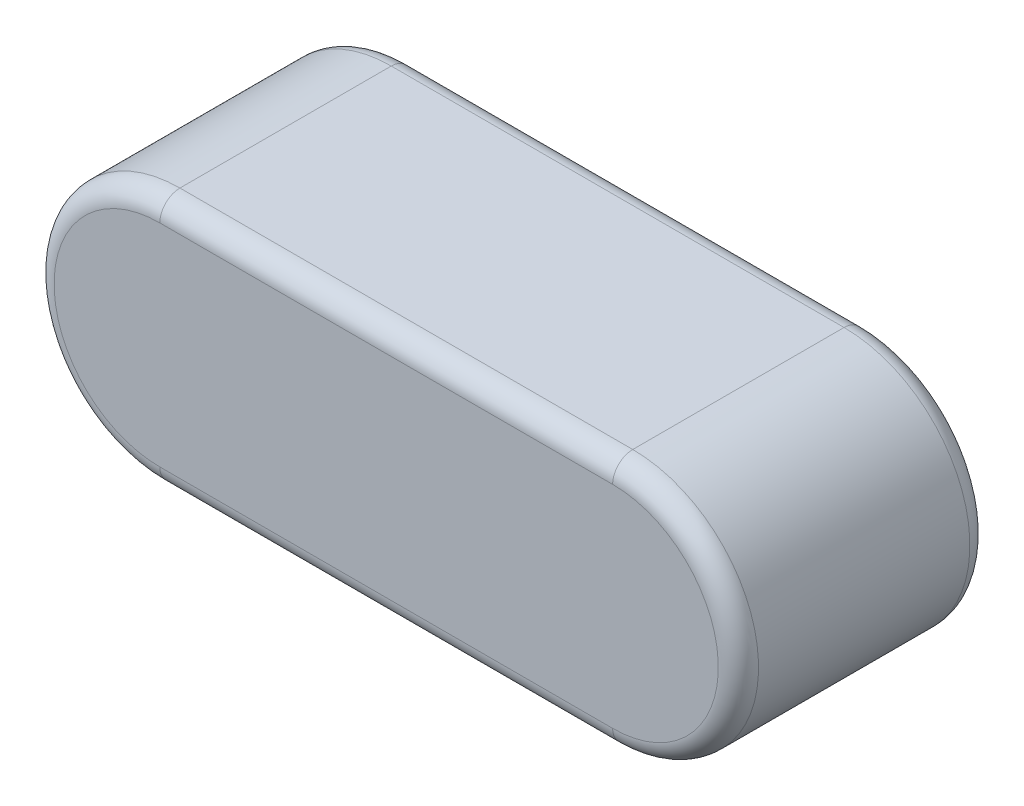
SolidWorks part; units mm, degrees
ref_plane "基准面1" through (0, 0, 0) normal (0, 0, 1) x (1, 0, 0)
ref_plane "基准面2" through (0, 0, 0) normal (0, 1, 0) x (1, 0, 0)
ref_plane "基准面3" through (0, 0, 0) normal (1, 0, 0) x (0, 0, -1)
sketch "尺寸草图" plane through (0, 0, 0) normal (0, 0, 1) x (1, 0, 0)
  line L0 (-7, 0) -> (7, 0) construction
  point P3 (-5, 0)
  point P4 (-0.4, 0)
  point P5 (0, 0)
  point P8 (-5, 0)
  point P11 (0, 0)
sketch "草图1" plane through (0, 0, 0) normal (0, 0, 1) x (1, 0, 0)
  line L0 (-28.0599, 0) -> (30.562, 0) construction
  line L1 (-4.5, 2.5) -> (4.5, 2.5)
  line L2 (-4.5, -2.5) -> (4.5, -2.5)
  line L3 (0, 2.9108) -> (0, -2.1805) construction
  arc A0 (-4.5, 2.5) -> (-4.5, -2.5) centre (-4.5, 0) ccw
  arc A1 (4.5, 2.5) -> (4.5, -2.5) centre (4.5, 0) cw
extrude "基体-拉伸" add sketch "草图1" along normal blind 5
fillet "圆角1" radius 0.4 8 edges at (7, 0, 5) (0, 2.5, 5) (-7, 0, 5) (0, 2.5, 0) (7, 0, 0) (0, -2.5, 0) (-7, 0, 0) (0, -2.5, 5)
equation "\"D3@草图1\" = \"L@尺寸草图\""
equation "\"D1@草图1\" = \"b@尺寸草图\" / 2"
equation "\"D1@圆角1\" = \"r@尺寸草图\""
equation "\"D1@基体-拉伸\" = \"h@尺寸草图\""
